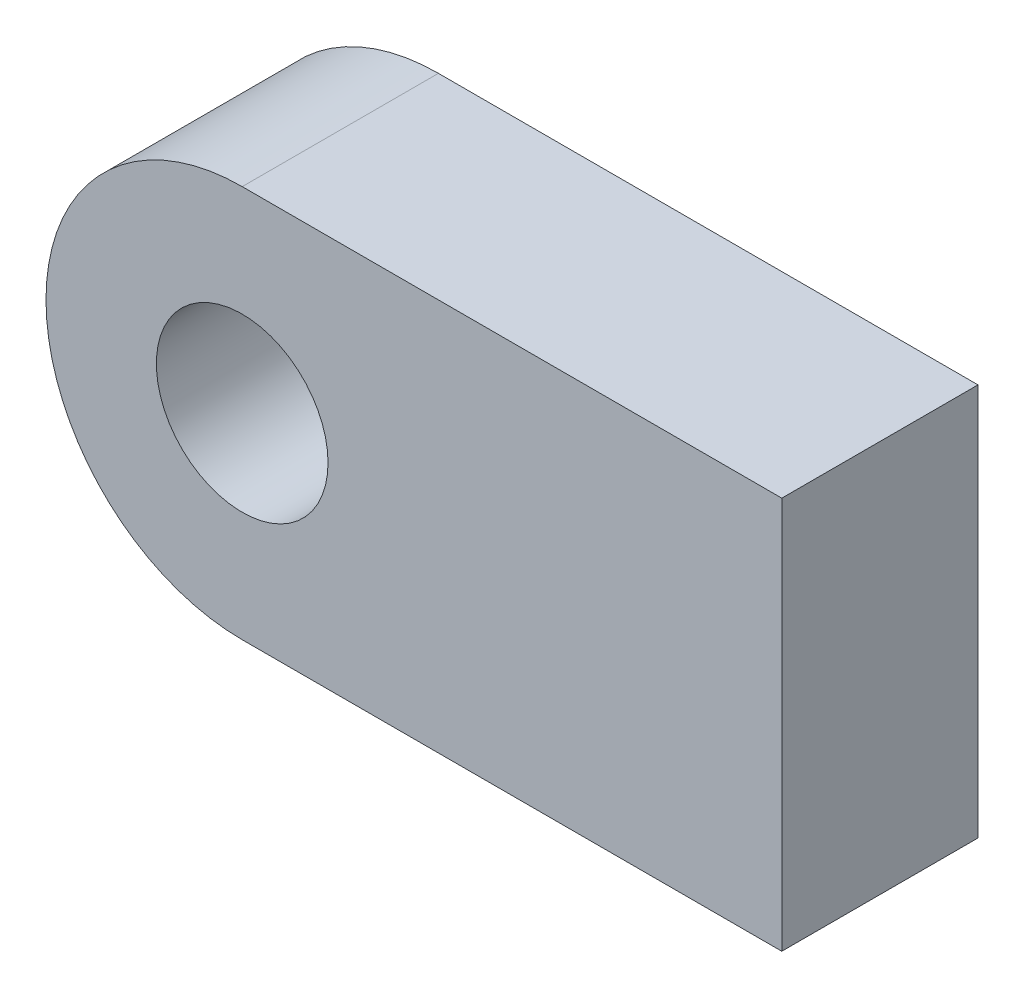
SolidWorks part; units mm, degrees
ref_plane "Front Plane" through (0, 0, 0) normal (0, 0, 1) x (1, 0, 0)
ref_plane "Top Plane" through (0, 0, 0) normal (0, 1, 0) x (1, 0, 0)
ref_plane "Right Plane" through (0, 0, 0) normal (1, 0, 0) x (0, 0, -1)
other "Configuration Table"
sketch "Sketch1" plane through (0, 0, 0) normal (0, 0, 1) x (1, 0, 0)
  line L0 (0, 8) -> (22, 8)
  line L1 (22, 8) -> (22, -8)
  line L2 (22, -8) -> (0, -8)
  circle A0 centre (0, 0) radius 3.5
  arc A1 (0, 8) -> (0, -8) centre (0, 0) ccw
  dimension "D1" = 7
  dimension "D2" = 16
  dimension "D3" = 22
extrude "Boss-Extrude1" add sketch "Sketch1" along normal blind 8
